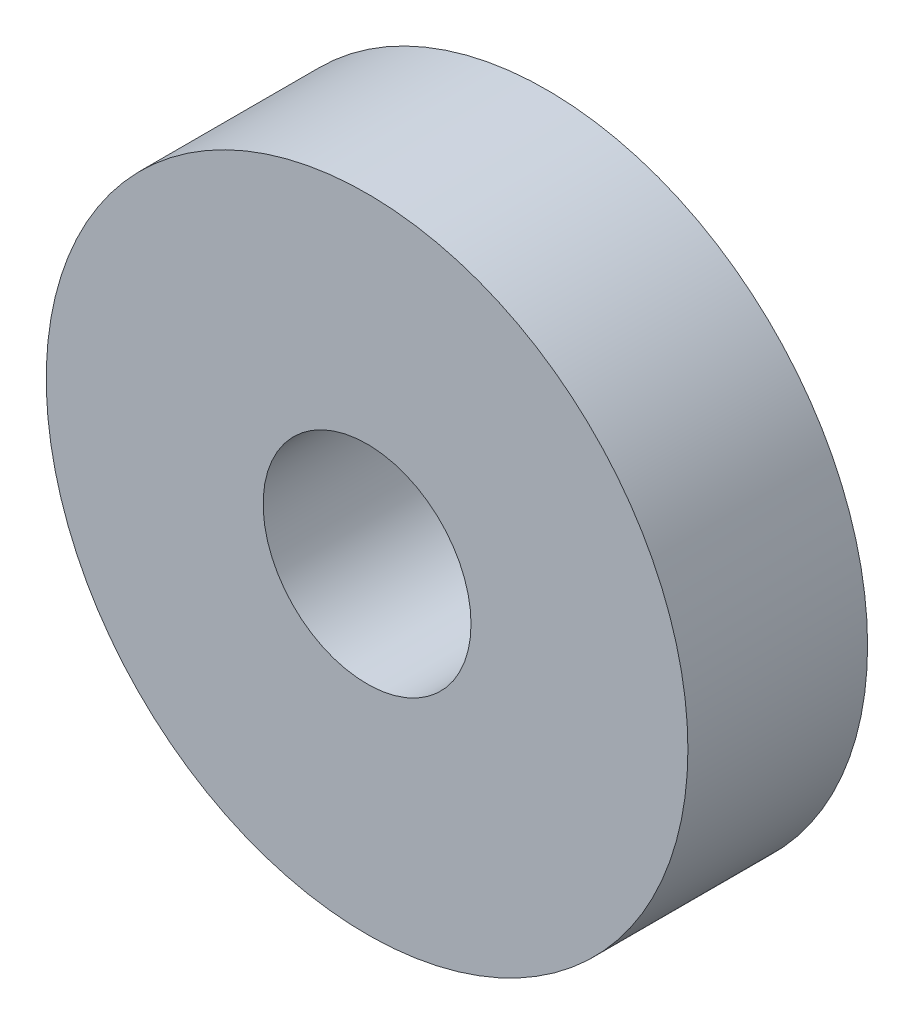
from build123d import *

# Parameters (mm, degrees)
SKETCH_1_R      = 25
SKETCH_1_R_2    = 8.1
EXTRUDE_1_DEPTH = 7


with BuildPart() as part:
    # 草图1 → 凸台-拉伸1 (new, symmetric)
    with BuildSketch(Plane.XY):
        Circle(SKETCH_1_R)
        Circle(SKETCH_1_R_2, mode=Mode.SUBTRACT)
    extrude(amount=EXTRUDE_1_DEPTH, both=True)


solid = part.part
